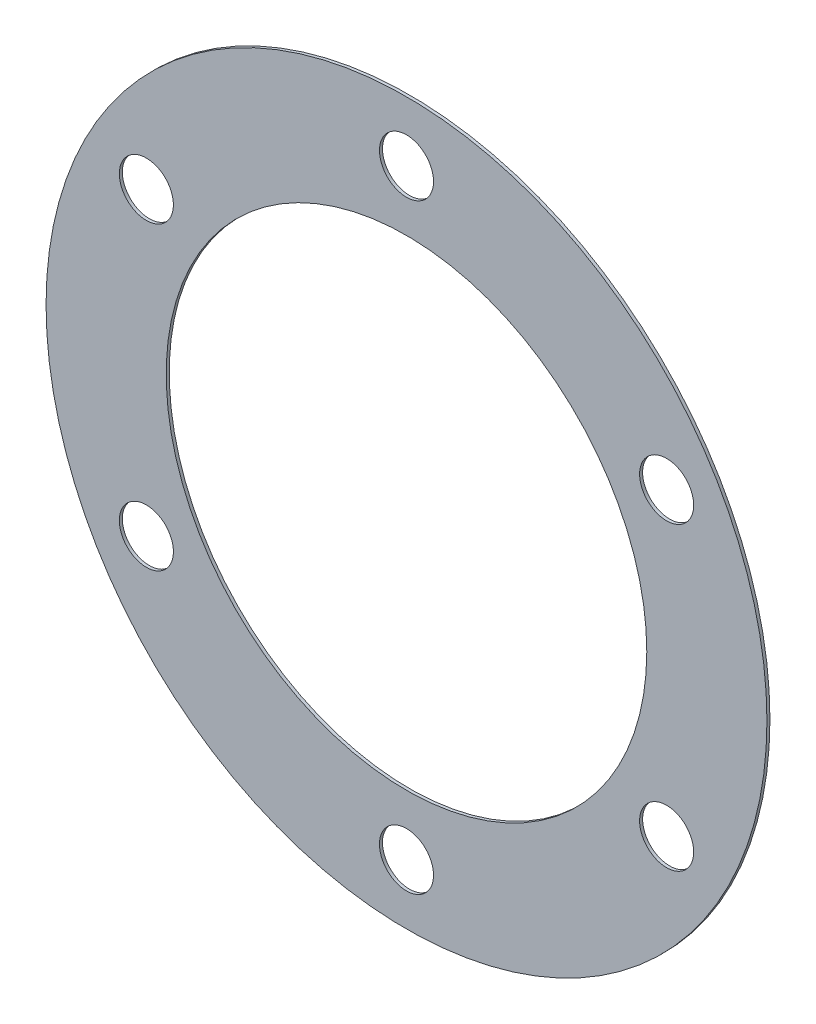
from build123d import *

# Parameters (mm, degrees)
SKETCH1_R           = 60
SKETCH1_R_2         = 40
BOSS_EXTRUDE1_DEPTH = 0.5
SKETCH2_R           = 4.5
CUT_EXTRUDE1_DEPTH  = 85.854286869
CIRPATTERN1_COUNT   = 6


with BuildPart() as part:
    # Sketch1 → Boss-Extrude1 (new body)
    with BuildSketch(Plane.XY):
        Circle(SKETCH1_R)
        Circle(SKETCH1_R_2, mode=Mode.SUBTRACT)
    extrude(amount=BOSS_EXTRUDE1_DEPTH)

    # Sketch2 → Cut-Extrude1 (cut, through all)
    with BuildSketch(Plane.XY.offset(0.5)):
        with Locations((0, 50)):
            Circle(SKETCH2_R)
    cut_extrude1 = extrude(amount=-CUT_EXTRUDE1_DEPTH, mode=Mode.SUBTRACT)

    # CirPattern1: Cut-Extrude1 ×6 about axis
    cirpattern1_axis = Axis((0, 0, 0), (0, 0, 1))
    for i in range(1, CIRPATTERN1_COUNT):
        add(cut_extrude1.rotate(cirpattern1_axis, i * 360 / CIRPATTERN1_COUNT), mode=Mode.SUBTRACT)


solid = part.part
